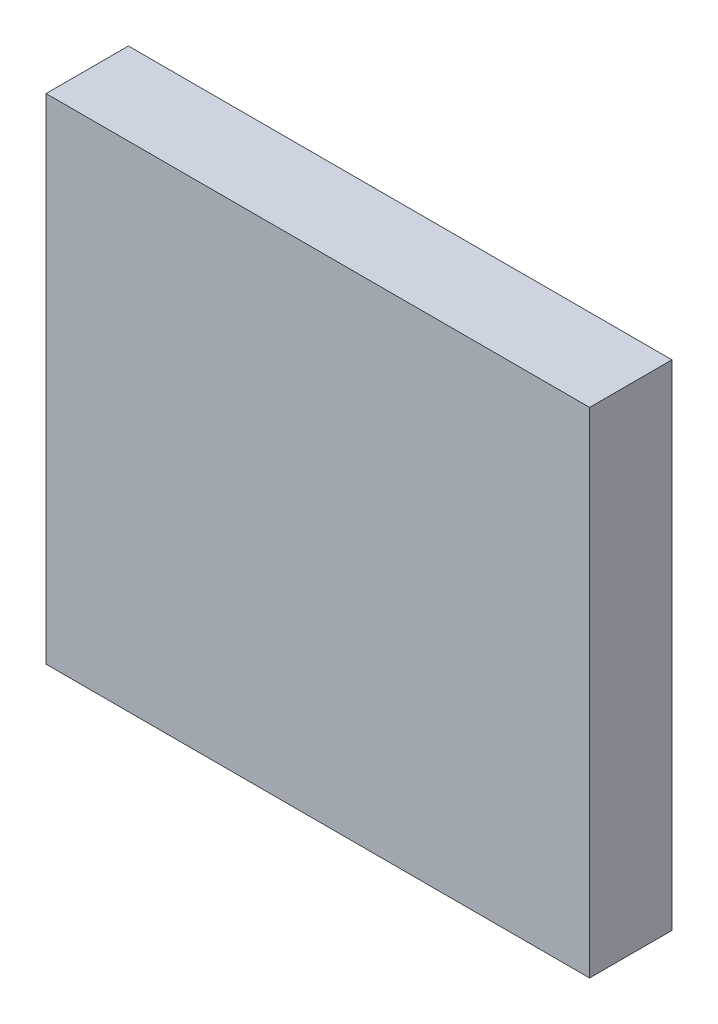
from build123d import *

# Parameters (mm, degrees)
SKETCH1_W           = 132
SKETCH1_H           = 120
BOSS_EXTRUDE1_DEPTH = 20


with BuildPart() as part:
    # Sketch1 → Boss-Extrude1 (new body)
    with BuildSketch(Plane.XY):
        with Locations((66, 60)):
            Rectangle(SKETCH1_W, SKETCH1_H)
    extrude(amount=BOSS_EXTRUDE1_DEPTH)


solid = part.part
